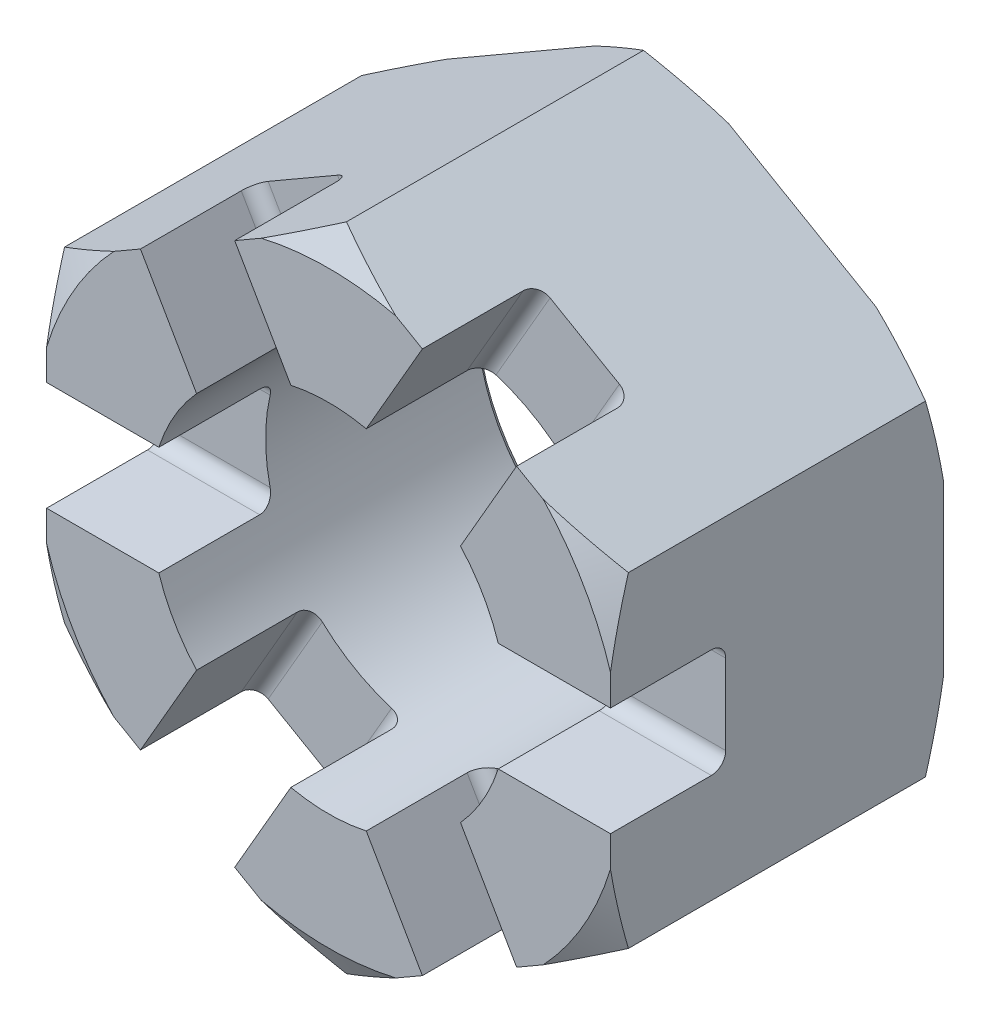
SolidWorks part; units mm, degrees
ref_plane "基准面1" through (0, 0, 0) normal (0, 0, 1) x (1, 0, 0)
ref_plane "基准面2" through (0, 0, 0) normal (0, 1, 0) x (1, 0, 0)
ref_plane "基准面3" through (0, 0, 0) normal (1, 0, 0) x (0, 0, -1)
sketch "尺寸草图" plane through (0, 0, 0) normal (0, 0, 1) x (1, 0, 0)
  line L0 (0, 0) -> (46, 0) construction
  line L1 (50.85, 0) -> (83.25, 0) construction
  line L2 (83.25, 0) -> (125.95, 0) construction
  line L3 (-26.5714, 0) -> (2, 0) construction
  line L4 (0, 0) -> (50.85, 0) construction
  point P3 (30, 0)
  point P4 (2, 0)
  point P5 (50.85, 0)
  point P6 (28.6, 0)
  point P8 (46, 0)
  point P15 (70.45, 0)
  point P16 (91.75, 0)
  dimension "D1" = 28.5714
  dimension "D" = 30
  dimension "P" = 2
  dimension "e(最小)" = 50.85
  dimension "m(最大)" = 28.6
  dimension "s(最大)" = 46
  dimension "da" = 32.4
  dimension "dw" = 42.7
  dimension "w(最大)" = 19.6
  dimension "n(最大)" = 8.5
sketch "草图1" plane through (0, 0, 0) normal (0, 0, 1) x (1, 0, 0)
  line L0 (-22.0187, 0) -> (22.0187, 0) construction
  line L1 (0, 25.425) -> (0, -25.425) construction
  line L3 (0, 25.425) -> (-22.0187, 12.7125)
  line L4 (-22.0187, 12.7125) -> (-22.0187, -12.7125)
  line L5 (-22.0187, -12.7125) -> (0, -25.425)
  line L6 (0, -25.425) -> (22.0187, -12.7125)
  line L7 (22.0187, -12.7125) -> (22.0187, 12.7125)
  line L8 (22.0187, 12.7125) -> (0, 25.425)
  circle A0 centre (0, 0) radius 22.0187 construction
  circle A1 centre (0, 0) radius 13.9175
  dimension "D" = 27.835
  dimension "e" = 50.85
extrude "基体-拉伸" add sketch "草图1" along normal blind 26
cosmetic thread "装饰螺纹线1" parameters "D2"=30
sketch "草图2" plane through (0, 0, 0) normal (0, 0, -1) x (-1, 0, 0)
  circle A0 centre (0, 0) radius 23
  circle A1 centre (0, 0) radius 13.9175 construction
  dimension "s" = 46
extrude "切除-拉伸1" cut sketch "草图2" against normal through all draft 60 flip side to cut
sketch "草图3" plane through (0, 0, 26) normal (0, 0, 1) x (1, 0, 0)
  circle A0 centre (0, 0) radius 23
  dimension "D1" = 46
extrude "切除-拉伸2" cut sketch "草图3" against normal through all draft 60 flip side to cut
sketch "草图6" plane through (22.0187, 0, 0) normal (1, 0, 0) x (0, 0, -1)
  line L0 (-14.9451, 0) -> (3.4921, 0) construction
  line L1 (-26, 0) -> (0, 0) construction
  line L3 (-26, -6.6466) -> (-26, 6.6466) construction
  line L4 (-26, -4.25) -> (-26, 4.25)
  line L5 (-26, 4.25) -> (-18.125, 4.25)
  line L6 (-17, -3.125) -> (-17, 3.125)
  line L8 (-26, -4.25) -> (-18.125, -4.25)
  arc A0 (-18.125, 4.25) -> (-17, 3.125) centre (-18.125, 3.125) cw
  arc A1 (-18.125, -4.25) -> (-17, -3.125) centre (-18.125, -3.125) ccw
  point P14 (-17, 4.25)
  point P17 (-17, -4.25)
  dimension "D1" = 1.125
  dimension "D2" = 9
  dimension "n" = 4.25
extrude "切除-拉伸3" cut sketch "草图6" against normal through all
pattern_circular "阵列(圆周)1" count 3 over 360 about axis through (0, 0, 0) along (0, 0, 1) of "切除-拉伸3"
chamfer "倒角1" distance 0.4786 angle 45 1 edges at (13.9175, 0, 0)
